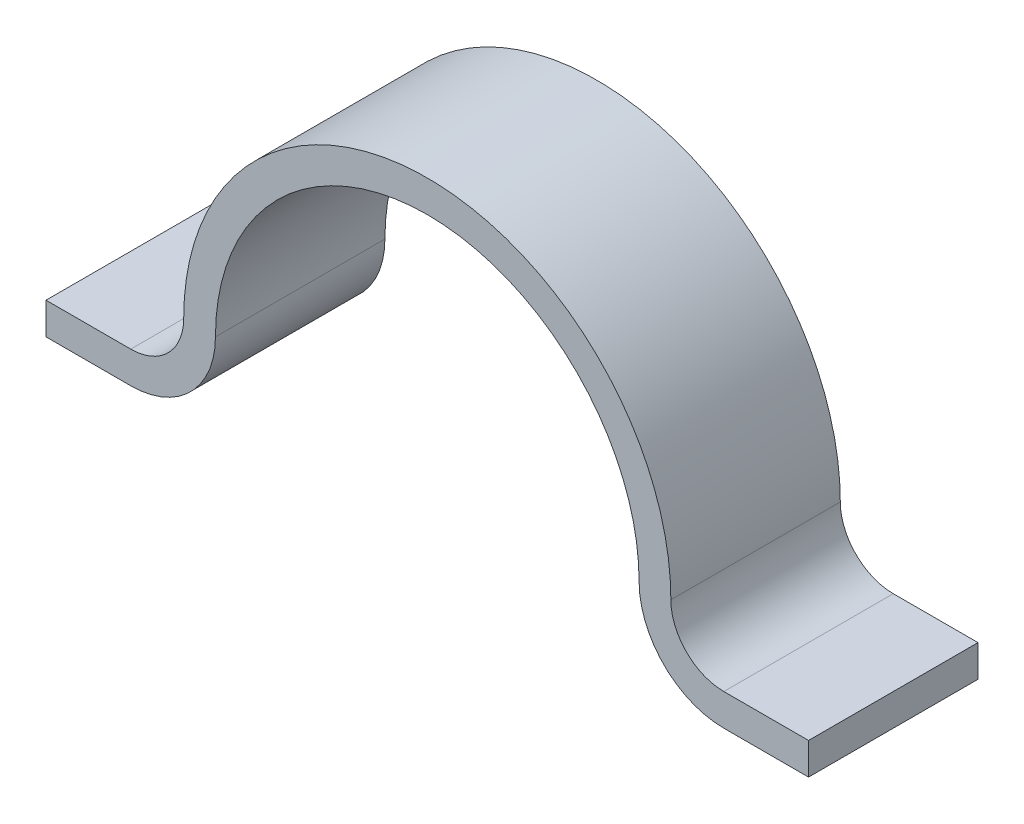
from build123d import *

# Parameters (mm, degrees)
BOSS_EXTRUDE1_DEPTH = 12.7


with BuildPart() as part:
    # Sketch1 → Boss-Extrude1 (new, symmetric)
    with BuildSketch(Plane.XY):
        with BuildLine():
            Line((57.15, 0), (57.15, 4.7625))
            Line((57.15, 4.7625), (44.45, 4.7625))
            ThreePointArc((44.45, 4.7625), (38.837339924, 7.087339924), (36.5125, 12.7))
            ThreePointArc((36.5125, 12.7), (0, 49.2125), (-36.5125, 12.7))
            ThreePointArc((-36.5125, 12.7), (-38.837339924, 7.087339924), (-44.45, 4.7625))
            Line((-44.45, 4.7625), (-57.15, 4.7625))
            Line((-57.15, 4.7625), (-57.15, 0))
            Line((-57.15, 0), (-44.45, 0))
            ThreePointArc((-44.45, 0), (-35.469743879, 3.719743879), (-31.75, 12.7))
            ThreePointArc((-31.75, 12.7), (0, 44.45), (31.75, 12.7))
            ThreePointArc((31.75, 12.7), (35.469743879, 3.719743879), (44.45, 0))
            Line((44.45, 0), (57.15, 0))
        make_face()
    extrude(amount=BOSS_EXTRUDE1_DEPTH, both=True)


solid = part.part
